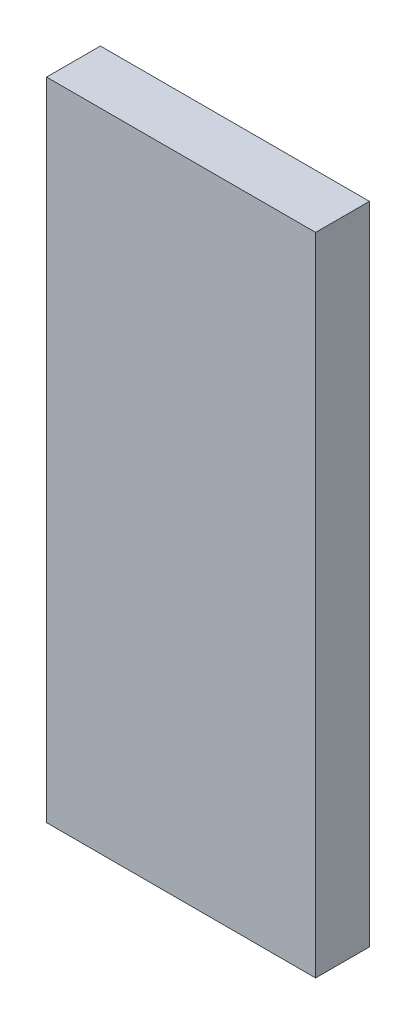
from build123d import *

# Parameters (mm, degrees)
SKETCH1_W           = 50
SKETCH1_H           = 120
BOSS_EXTRUDE1_DEPTH = 5


with BuildPart() as part:
    # Sketch1 → Boss-Extrude1 (new, symmetric)
    with BuildSketch(Plane.XY):
        Rectangle(SKETCH1_W, SKETCH1_H)
    extrude(amount=BOSS_EXTRUDE1_DEPTH, both=True)


solid = part.part
